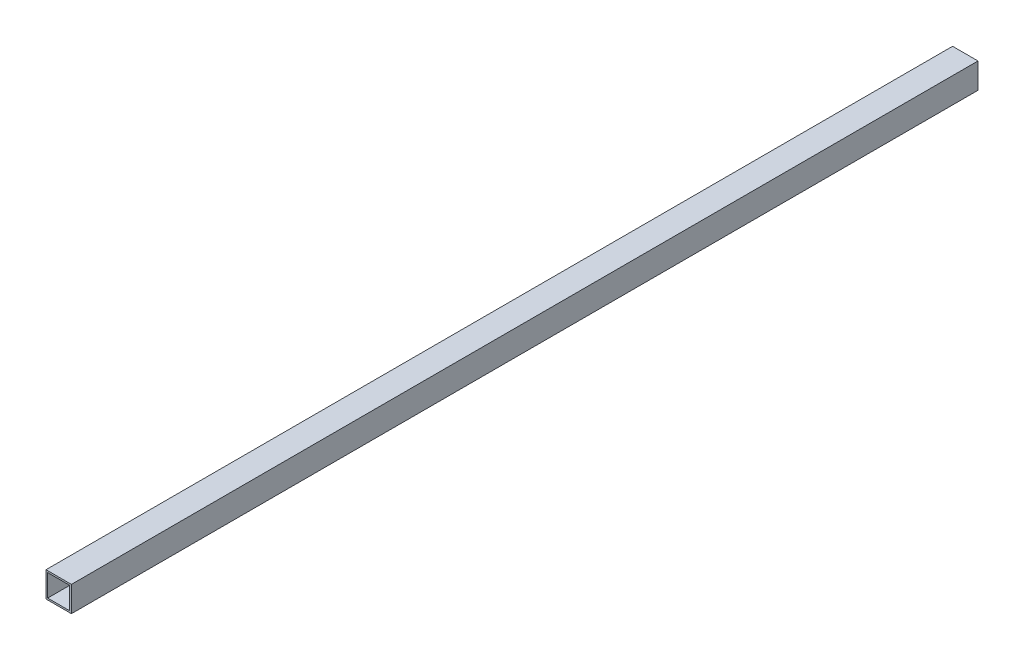
SolidWorks part; units mm, degrees
ref_plane "前视基准面" through (0, 0, 0) normal (0, 0, 1) x (1, 0, 0)
ref_plane "上视基准面" through (0, 0, 0) normal (0, 1, 0) x (1, 0, 0)
ref_plane "右视基准面" through (0, 0, 0) normal (1, 0, 0) x (0, 0, -1)
sketch "草图1" plane through (0, 0, 0) normal (0, 0, 1) x (1, 0, 0)
  line L0 (13, 13) -> (-13, 13)
  line L1 (15, -15) -> (-15, -15)
  line L2 (15, -15) -> (15, 15)
  line L3 (15, 15) -> (-15, 15)
  line L4 (-15, -15) -> (-15, 15)
  line L5 (15, -15) -> (-15, 15) construction
  line L6 (15, 15) -> (-15, -15) construction
  line L7 (-13, -13) -> (-13, 13)
  line L8 (13, -13) -> (-13, -13)
  line L9 (13, -13) -> (13, 13)
  point P0 (0, 0)
  dimension "D1" = 30
  dimension "D2" = 2
extrude "凸台-拉伸1" add sketch "草图1" along normal blind 1070
sketch "草图2" plane through (0, 0, 1070) normal (0, 0, 1) x (1, 0, 0)
  circle A0 centre (0, 0) radius 5.4673
